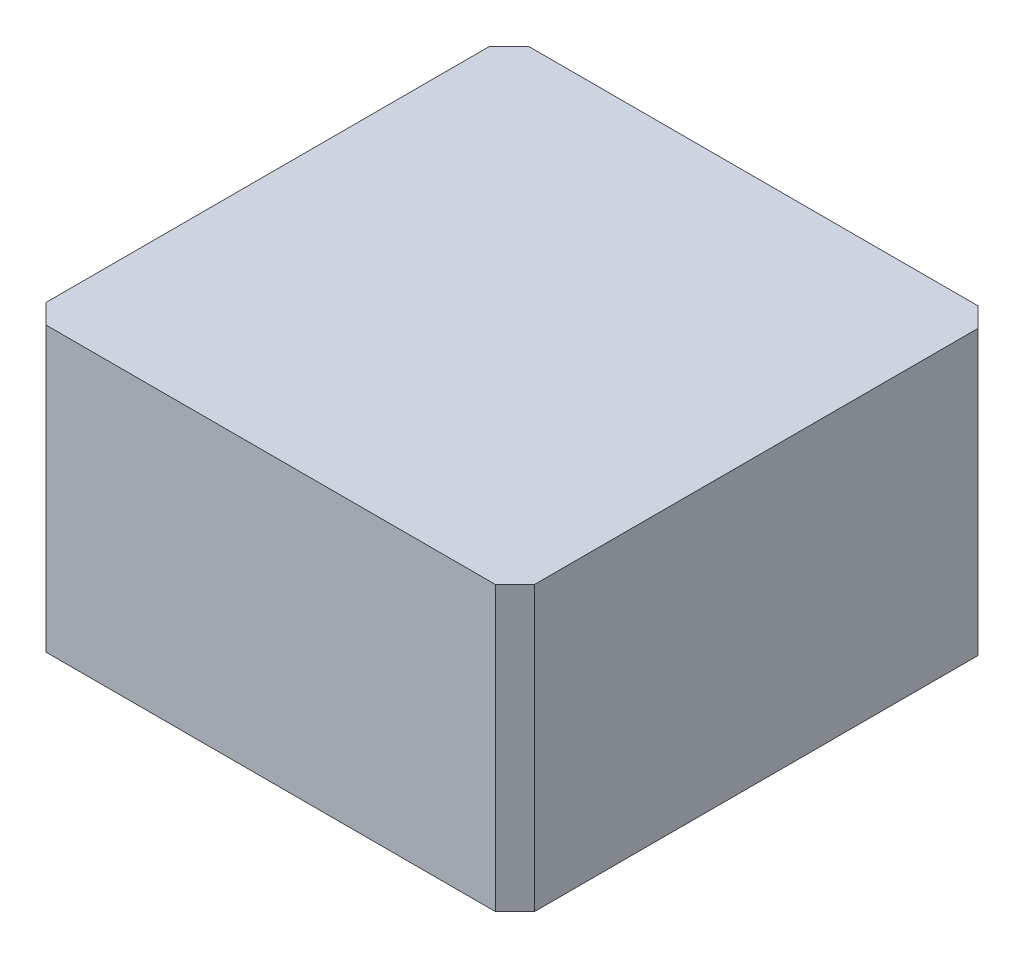
SolidWorks part; units mm, degrees
ref_plane "Front Plane" through (0, 0, 0) normal (0, 0, 1) x (1, 0, 0)
ref_plane "Top Plane" through (0, 0, 0) normal (0, 1, 0) x (1, 0, 0)
ref_plane "Right Plane" through (0, 0, 0) normal (1, 0, 0) x (0, 0, -1)
other "Configuration Table"
sketch "Sketch1" plane through (0, 0, 0) normal (0, 1, 0) x (1, 0, 0)
  line L1 (-125, -123.5) -> (125, -123.5)
  line L2 (-125, -123.5) -> (-125, 123.5)
  line L3 (-125, 123.5) -> (125, 123.5)
  line L4 (125, -123.5) -> (125, 123.5)
  line L5 (-125, -123.5) -> (125, 123.5) construction
  line L6 (-125, 123.5) -> (125, -123.5) construction
  point P0 (0, 0)
  dimension "D1" = 247
  dimension "D2" = 250
extrude "Boss-Extrude1" add sketch "Sketch1" along normal blind 145
sketch "Sketch2" plane through (0, 0, 0) normal (0, -1, 0) x (1, 0, 0)
  line L0 (0, 123.5) -> (0, -123.5) construction
  line L5 (-125, 123.5) -> (125, 123.5) construction
  line L6 (125, -123.5) -> (-125, -123.5) construction
  line L7 (-125, 123.5) -> (0, 123.5) construction
  line L8 (-100, 125) -> (-100, -123.5) construction
  line L9 (-125, 0) -> (125, 0) construction
  line L10 (-125, -123.5) -> (-125, 123.5) construction
  line L11 (125, 123.5) -> (125, -123.5) construction
  line L12 (-122.5, -27.5) -> (-77.5, -72.5) construction
  line L17 (-122.5, 72.5) -> (-77.5, 72.5)
  line L18 (-122.5, 72.5) -> (-122.5, 27.5)
  line L19 (-201.75, 50) -> (125, 50) construction
  line L20 (-122.5, 27.5) -> (-77.5, 27.5)
  line L21 (-77.5, 72.5) -> (-77.5, 27.5)
  line L22 (-122.5, 72.5) -> (-77.5, 27.5) construction
  line L23 (-122.5, 27.5) -> (-77.5, 72.5) construction
  line L24 (-122.5, -72.5) -> (-77.5, -27.5) construction
  line L25 (-77.5, -72.5) -> (-77.5, -27.5)
  line L26 (-122.5, -27.5) -> (-77.5, -27.5)
  line L27 (-122.5, -72.5) -> (-122.5, -27.5)
  line L28 (-122.5, -72.5) -> (-77.5, -72.5)
  point P16 (-100, 50)
  point P27 (-100, -50)
  dimension "D1" = 45
  dimension "D2" = 45
  dimension "D3" = 50
  dimension "D4" = 100
chamfer "Chamfer1" distance 10 angle 45 4 edges at (125, 72.5, 123.5) (125, 72.5, -123.5) (-125, 72.5, -123.5) (-125, 72.5, 123.5)
sketch "Sketch3" plane through (0, 0, 0) normal (0, -1, 0) x (1, 0, 0)
  line L0 (-101, -100) -> (-101, 100)
  line L1 (-106, -105) -> (106, -105)
  line L2 (-106, -105) -> (-106, 105)
  line L3 (-106, 105) -> (106, 105)
  line L4 (106, -105) -> (106, 105)
  line L5 (-106, -105) -> (106, 105) construction
  line L6 (-106, 105) -> (106, -105) construction
  line L7 (-101, 100) -> (101, 100)
  line L8 (101, -100) -> (101, 100)
  line L9 (-101, -100) -> (101, -100)
  point P0 (0, 0)
  dimension "D1" = 212
  dimension "D2" = 210
  dimension "D3" = 5
extrude "Cut-Extrude2" cut sketch "Sketch3" against normal blind 1
